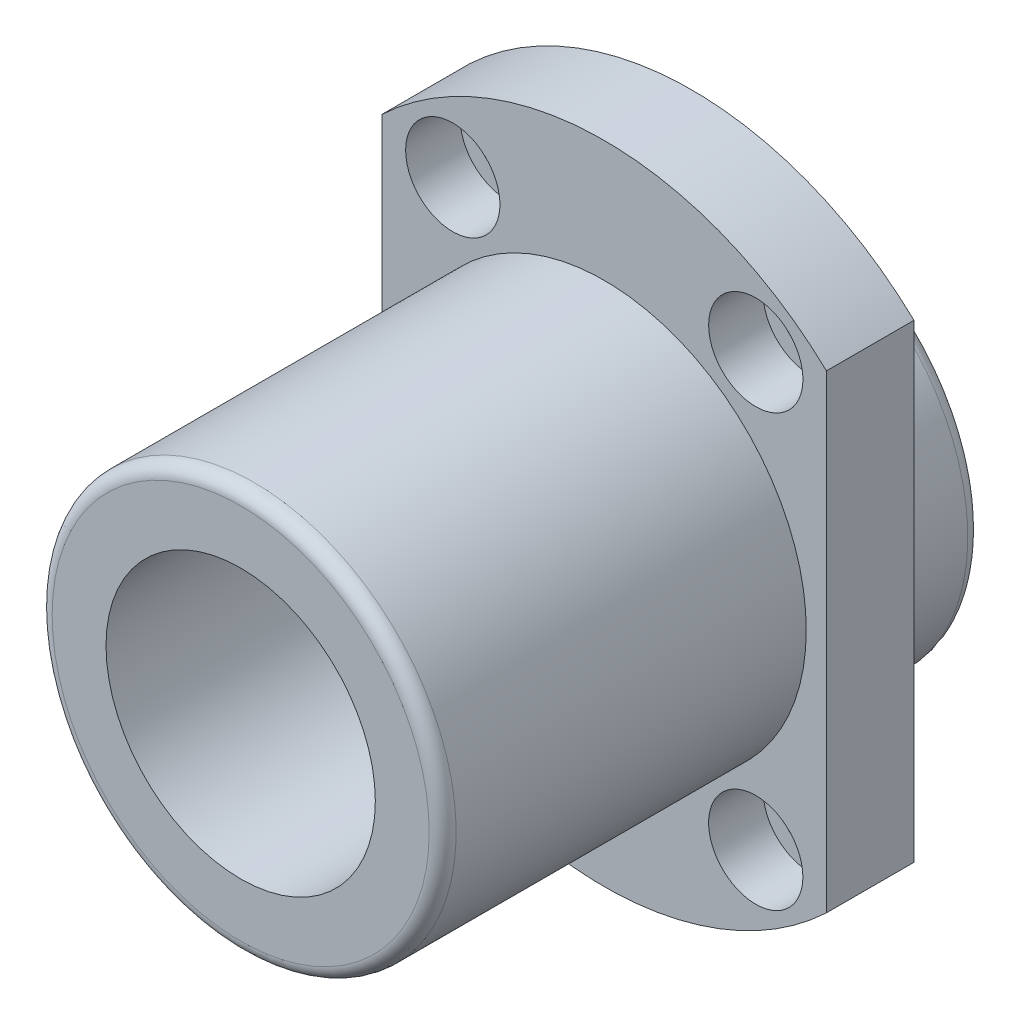
SolidWorks part; units mm, degrees
ref_plane "前视基准面" through (0, 0, 0) normal (0, 0, 1) x (1, 0, 0)
ref_plane "上视基准面" through (0, 0, 0) normal (0, 1, 0) x (1, 0, 0)
ref_plane "右视基准面" through (0, 0, 0) normal (1, 0, 0) x (0, 0, -1)
sketch "草图1" plane through (0, 0, 0) normal (1, 0, 0) x (0, 0, -1)
  line L0 (-67, 28) -> (-67, 20)
  line L1 (-67, 20) -> (13, 20)
  line L2 (13, 20) -> (13, 28)
  line L3 (11, 30) -> (-65, 30)
  line L4 (13, 0) -> (-67, 0) construction
  arc A0 (13, 28) -> (11, 30) centre (11, 28) ccw
  arc A1 (-65, 30) -> (-67, 28) centre (-65, 28) ccw
revolve "旋转1" add sketch "草图1" angle 360 about L4
sketch "草图2" plane through (0, 0, 0) normal (0, 0, 1) x (1, 0, 0)
  line L0 (-33, 34.8569) -> (-33, -34.8569)
  line L1 (33, -34.8569) -> (33, 34.8569)
  arc A0 (-33, -34.8569) -> (33, -34.8569) centre (0, 0) ccw
  arc A1 (33, 34.8569) -> (-33, 34.8569) centre (0, 0) ccw
  circle A2 centre (0, 0) radius 30
extrude "凸台-拉伸1" add sketch "草图2" along normal blind 13
ref_plane "基准面1" through (-22.5, 0, 0) normal (1, 0, 0) x (0, 0, -1)
sketch "草图3" plane through (-22.5, 0, 0) normal (1, 0, 0) x (0, 0, -1)
  line L0 (-13, 32) -> (-13, 39)
  line L1 (-13, 39) -> (-4.9, 39)
  line L2 (-4.9, 39) -> (-4.9, 36.5)
  line L3 (-4.9, 36.5) -> (0, 36.5)
  line L4 (0, 36.5) -> (0, 32)
  line L5 (0, 32) -> (-13, 32)
  line L6 (0, 32) -> (-13, 32) construction
revolve "切除-旋转1" cut sketch "草图3" angle 360 about L6
sketch "草图4" plane through (-22.5, 0, 0) normal (1, 0, 0) x (0, 0, -1)
  line L0 (0, -32) -> (0, -36.5)
  line L1 (0, -36.5) -> (-4.9, -36.5)
  line L2 (-4.9, -36.5) -> (-4.9, -39)
  line L3 (-4.9, -39) -> (-13, -39)
  line L4 (-13, -39) -> (-13, -32)
  line L5 (-13, -32) -> (0, -32)
  line L6 (-13, -32) -> (0, -32) construction
revolve "切除-旋转2" cut sketch "草图4" angle 360 about L6
ref_plane "基准面2" through (22.5, 0, 0) normal (1, 0, 0) x (0, 0, -1)
sketch "草图5" plane through (22.5, 0, 0) normal (1, 0, 0) x (0, 0, -1)
  line L0 (-13, 32) -> (-13, 39)
  line L1 (-13, 39) -> (-4.9, 39)
  line L2 (-4.9, 39) -> (-4.9, 36.5)
  line L3 (-4.9, 36.5) -> (0, 36.5)
  line L4 (0, 36.5) -> (0, 32)
  line L5 (0, 32) -> (-13, 32)
  line L6 (0, 32) -> (-13, 32) construction
revolve "切除-旋转3" cut sketch "草图5" angle 360 about L6
sketch "草图6" plane through (22.5, 0, 0) normal (1, 0, 0) x (0, 0, -1)
  line L0 (0, -32) -> (0, -36.5)
  line L1 (0, -36.5) -> (-4.9, -36.5)
  line L2 (-4.9, -36.5) -> (-4.9, -39)
  line L3 (-4.9, -39) -> (-13, -39)
  line L4 (-13, -39) -> (-13, -32)
  line L5 (-13, -32) -> (0, -32)
  line L6 (-13, -32) -> (0, -32) construction
revolve "切除-旋转4" cut sketch "草图6" angle 360 about L6
other "冻结***"
